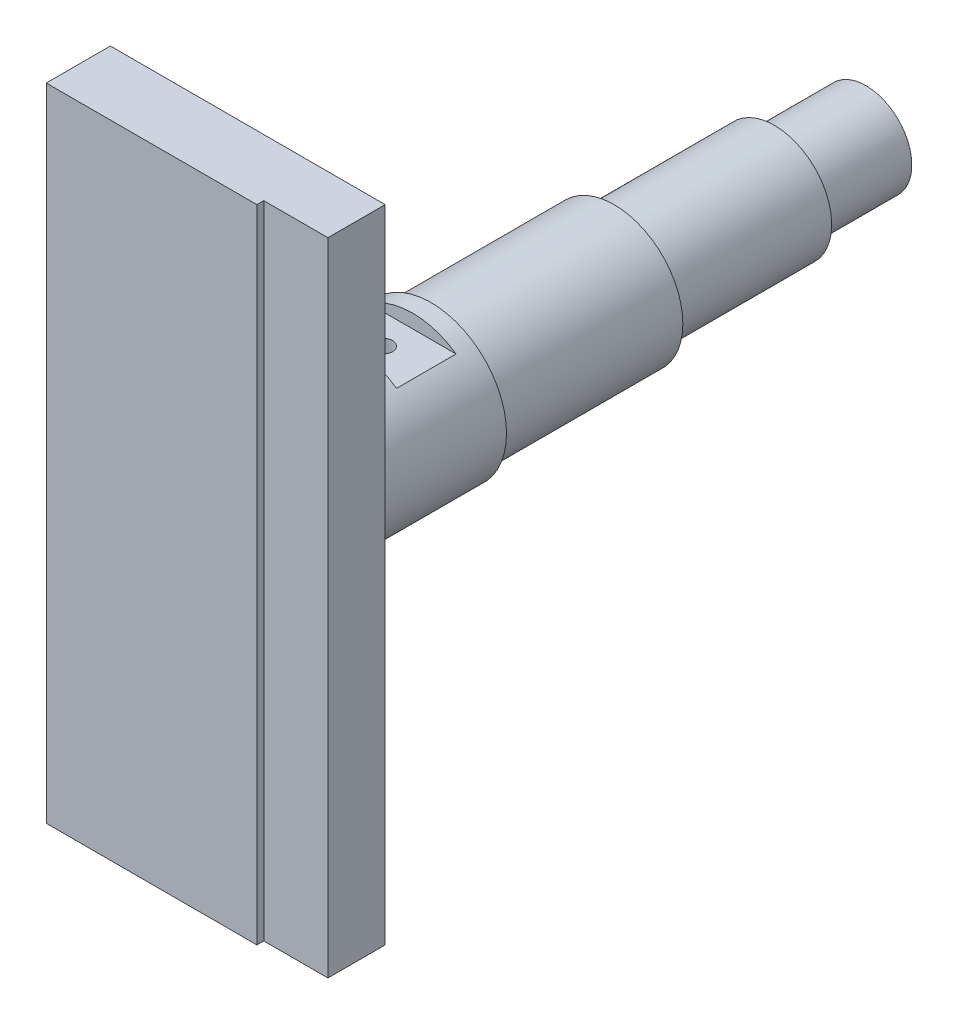
from build123d import *

# Parameters (mm, degrees)
SKETCH_1_R          = 15
EXTRUDE_1_DEPTH     = 40
SKETCH_2_R          = 16.5
EXTRUDE_2_DEPTH     = 40
SKETCH_3_R          = 12.5
EXTRUDE_3_DEPTH     = 35
SKETCH_4_R          = 10
EXTRUDE_4_DEPTH     = 20
SKETCH_5_W          = 60
SKETCH_5_H          = 140
EXTRUDE_5_DEPTH     = 14
SKETCH_6_W          = 14
SKETCH_6_H          = 140
CUT_EXTRUDE_1_DEPTH = 1.5
SKETCH_7_W          = 13
SKETCH_7_H          = 3
CUT_EXTRUDE_2_DEPTH = 10


with BuildPart() as part:
    # 草图1 → 凸台-拉伸1 (new body)
    with BuildSketch(Plane.XY):
        Circle(SKETCH_1_R)
    extrude(amount=EXTRUDE_1_DEPTH)

    # 草图2 → 凸台-拉伸2 (add)
    with BuildSketch(Plane.XY.offset(40)):
        Circle(SKETCH_2_R)
    extrude(amount=EXTRUDE_2_DEPTH)

    # 草图3 → 凸台-拉伸3 (add)
    with BuildSketch(Plane(origin=(0, 0, 0), x_dir=(-1, 0, 0), z_dir=(0, 0, -1))):
        Circle(SKETCH_3_R)
    extrude(amount=EXTRUDE_3_DEPTH)

    # 草图4 → 凸台-拉伸4 (add)
    with BuildSketch(Plane(origin=(0, 0, -35), x_dir=(-1, 0, 0), z_dir=(0, 0, -1))):
        Circle(SKETCH_4_R)
    extrude(amount=EXTRUDE_4_DEPTH)

    # 草图5 → 凸台-拉伸5 (add)
    with BuildSketch(Plane.XY.offset(80)):
        Rectangle(SKETCH_5_W, SKETCH_5_H)
    extrude(amount=EXTRUDE_5_DEPTH)

    # 草图6 → 切除-拉伸1 (cut)
    with BuildSketch(Plane.XY.offset(94)):
        with Locations((23, 0)):
            Rectangle(SKETCH_6_W, SKETCH_6_H)
    extrude(amount=-CUT_EXTRUDE_1_DEPTH, mode=Mode.SUBTRACT)

    # 草图7 → 切除-拉伸2 (cut, symmetric)
    with BuildSketch(Plane(origin=(0, 0, 0), x_dir=(0, 0, -1), z_dir=(1, 0, 0))):
        with Locations((-50.5, 15)):
            Rectangle(SKETCH_7_W, SKETCH_7_H)
    cut_extrude_2 = extrude(amount=CUT_EXTRUDE_2_DEPTH, both=True, mode=Mode.SUBTRACT)

    # 镜向1: 切除-拉伸2 across plane
    add(cut_extrude_2.mirror(Plane.ZX), mode=Mode.SUBTRACT)

    # 草图8 → M5 螺纹孔1 (revolve, cut)
    with BuildSketch(Plane(origin=(0, 13.5, 50.5), x_dir=(0, 0, 1), z_dir=(1, 0, 0))):
        Polygon((0, 0), (0, 11.2618073), (2.1, 10), (2.1, 0), align=None)
    hole_wizard_m5_1 = revolve(axis=Axis((0, 19.85, 50.5), (0, -1, 0)), mode=Mode.SUBTRACT)

    # 镜向2: M5 螺纹孔1 across plane
    add(hole_wizard_m5_1.mirror(Plane.ZX), mode=Mode.SUBTRACT)


solid = part.part
